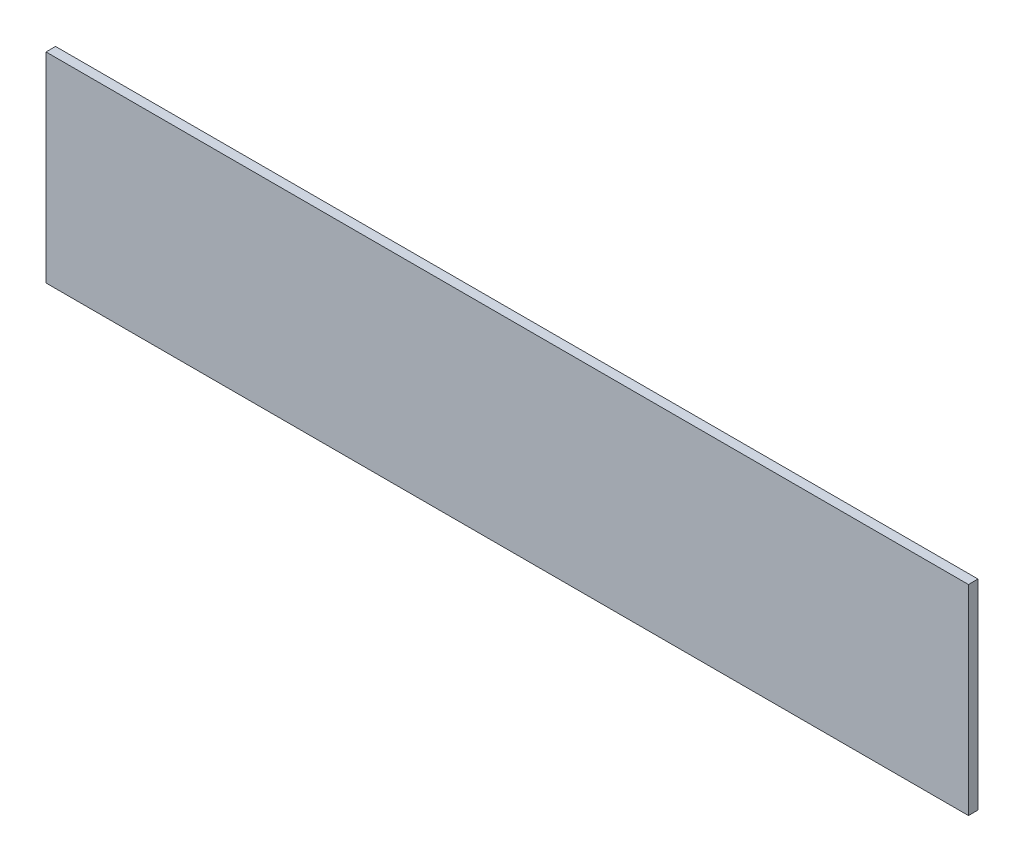
SolidWorks part; units mm, degrees
material "PMMA(有机玻璃)"
ref_plane "前视" through (0, 0, 0) normal (0, 0, 1) x (1, 0, 0)
ref_plane "上视" through (0, 0, 0) normal (0, 1, 0) x (1, 0, 0)
ref_plane "右视" through (0, 0, 0) normal (1, 0, 0) x (0, 0, -1)
sketch "草图1" plane through (0, 0, 0) normal (0, 0, 1) x (1, 0, 0)
  line L1 (-242, 52.5) -> (242, 52.5)
  line L2 (-242, 52.5) -> (-242, -52.5)
  line L3 (-242, -52.5) -> (242, -52.5)
  line L4 (242, 52.5) -> (242, -52.5)
  line L5 (-242, 52.5) -> (242, -52.5) construction
  line L6 (-242, -52.5) -> (242, 52.5) construction
  point P0 (0, 0)
  dimension "D1" = 105
  dimension "D2" = 484
extrude "凸台-拉伸1" add sketch "草图1" along normal blind 5
hole_wizard "M5 间隙孔1" positions "草图3" profile "草图2" hole size "M5" standard "GB"
sketch "草图3" plane through (0, 0, 5) normal (0, 0, 1) x (1, 0, 0)
  line L0 (-427.5, 273) -> (-427.5, -273) construction
  line L1 (-427.5, -273) -> (427.5, -273) construction
  line L2 (0, 273) -> (0, -273) construction
  line L3 (427.5, 273) -> (-427.5, 273) construction
  line L5 (-427.5, 0) -> (427.5, 0) construction
  line L6 (427.5, -273) -> (427.5, 273) construction
  point P0 (-375, -261)
  point P46 (415.5, 250)
  point P48 (-415.5, 250)
  point P58 (-125, -261)
  point P59 (125, -261)
  point P61 (-125, 261)
  point P62 (125, 261)
  point P64 (-375, 261)
  point P88 (375, -261)
  point P89 (375, 261)
  point P108 (415.5, 0)
  point P109 (-415.5, 0)
  point P110 (415.5, -250)
  point P111 (-415.5, -250)
  dimension "D1" = 12
  dimension "D2" = 12
  dimension "D5" = 3
  dimension "D3" = 12
  dimension "D6" = 4
  dimension "D4" = 2
sketch "草图2" plane through (-375, -261, 5) normal (1, 0, 0) x (0, -1, 0)
  line L0 (0, 0) -> (0, 5)
  line L1 (0, 5) -> (2.75, 5)
  line L2 (2.75, 5) -> (2.75, 0)
  line L5 (2.75, 0) -> (0, 0)
  line L11 (0, -6.35) -> (0, 107.95) construction
  dimension "通孔孔直径" = 5.5
  dimension "通孔孔深度" = 5
